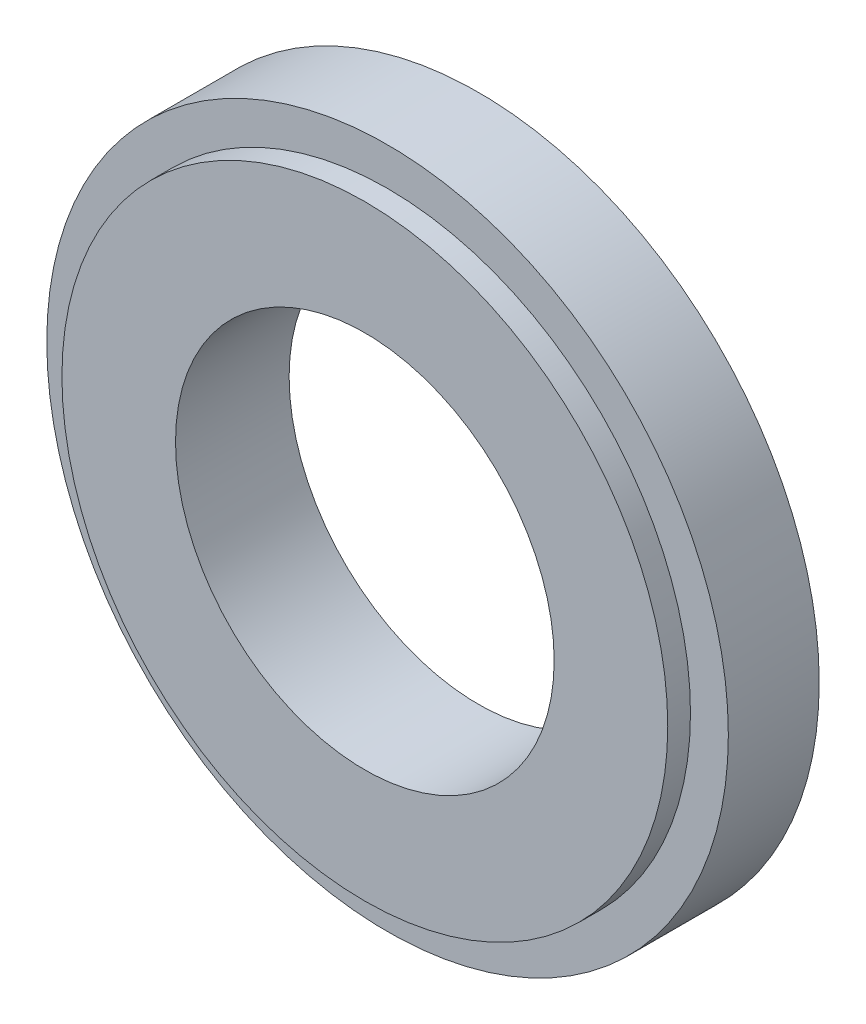
SolidWorks part; units mm, degrees
ref_plane "Front Plane" through (0, 0, 0) normal (0, 0, 1) x (1, 0, 0)
ref_plane "Top Plane" through (0, 0, 0) normal (0, 1, 0) x (1, 0, 0)
ref_plane "Right Plane" through (0, 0, 0) normal (1, 0, 0) x (0, 0, -1)
sketch "Sketch1" plane through (0, 0, 0) normal (0, 0, 1) x (1, 0, 0)
  circle A0 centre (0, 0) radius 45
  circle A1 centre (0, 0) radius 25
extrude "Boss-Extrude1" add sketch "Sketch1" along normal blind 12
sketch "Sketch2" plane through (0, 0, 12) normal (0, 0, 1) x (1, 0, 0)
  circle A0 centre (0, 0) radius 40
  circle A1 centre (0, 0) radius 25
extrude "Boss-Extrude2" add sketch "Sketch2" along normal blind 3
sketch "Sketch5" plane through (0, 0, 0) normal (0, 0, -1) x (-1, 0, 0)
  circle A1 centre (0, 37) radius 1.95
  circle A2 centre (32.0429, 18.5) radius 1.95
  circle A3 centre (32.0429, -18.5) radius 1.95
  circle A4 centre (0, -37) radius 1.95
  circle A5 centre (-32.0429, -18.5) radius 1.95
  circle A6 centre (-32.0429, 18.5) radius 1.95
  point P17 (0, 0)
  dimension "D1" = 6
hole_wizard "M4 Tapped Hole2" positions "3DSketch2" profile "Sketch6" tap size "M4" standard "Gb"
sketch3d "3DSketch2"
  point P0 (32.0429, 18.5, 0)
  point P3 (0, 37, 0)
  point P6 (-32.0429, 18.5, 0)
  point P9 (-32.0429, -18.5, 0)
  point P12 (0, -37, 0)
  point P15 (32.0429, -18.5, 0)
sketch "Sketch6" plane through (32.0429, 18.5, 0) normal (1, 0, 0) x (0, 1, 0)
  line L0 (0, 0) -> (0, 11.0914)
  line L1 (0, 11.0914) -> (1.65, 10.1)
  line L2 (1.65, 10.1) -> (1.65, 0)
  line L5 (1.65, 0) -> (0, 0)
  line L10 (0, 11.0914) -> (-1.65, 10.1) construction
  line L11 (0, -6.35) -> (0, 107.95) construction
  dimension "螺纹孔钻头直径" = 3.3
  dimension "螺纹孔钻头深度" = 10.1
  dimension "导头角度" = 118
cosmetic thread "Cosmetic Thread7" parameters "D1"=8, "D2"=4
cosmetic thread "Cosmetic Thread8" parameters "D1"=8, "D2"=4
cosmetic thread "Cosmetic Thread9" parameters "D1"=8, "D2"=4
cosmetic thread "Cosmetic Thread10" parameters "D1"=8, "D2"=4
cosmetic thread "Cosmetic Thread11" parameters "D1"=8, "D2"=4
cosmetic thread "Cosmetic Thread12" parameters "D1"=8, "D2"=4
